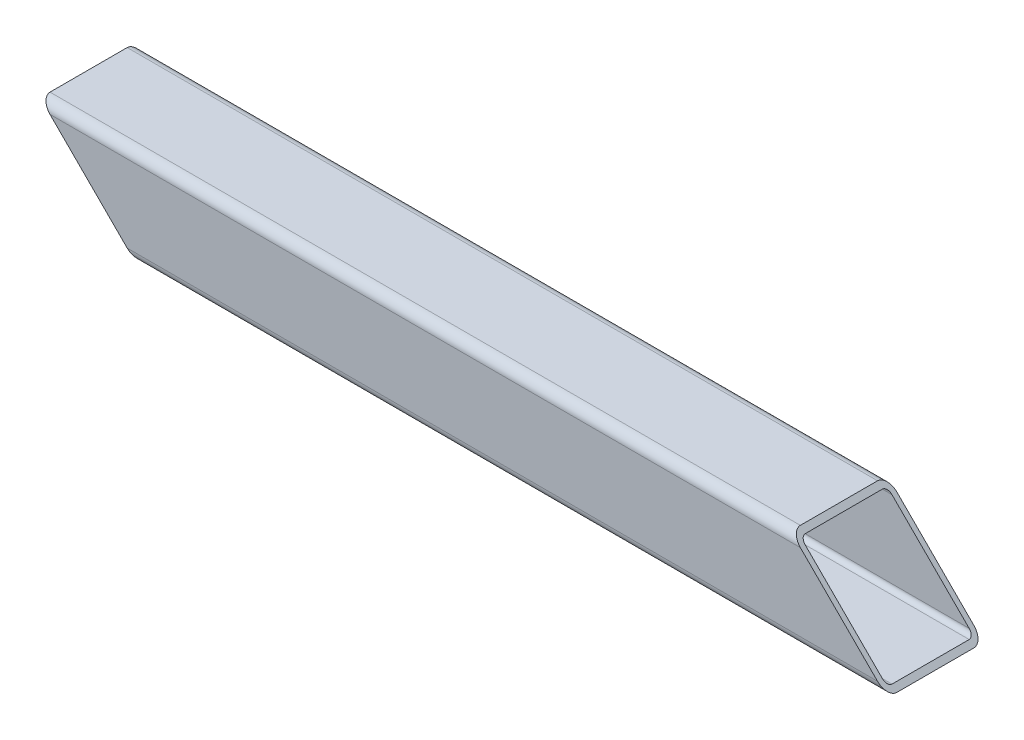
from build123d import *

# Parameters (mm, degrees)
F_100_X_100_X_5_1_DEPTH = 900
CUT_EXTRUDE_1_DEPTH     = 100


with BuildPart() as part:
    # Sketch1 → 方形管 100 X 100 X 5(1) (new body)
    with BuildSketch(Plane(origin=(0, 0, 0), x_dir=(0, 0, -1), z_dir=(1, 0, 0))):
        with BuildLine():
            Line((-40, -50), (40, -50))
            ThreePointArc((40, -50), (47.071067812, -47.071067812), (50, -40))
            Line((50, -40), (50, 40))
            ThreePointArc((50, 40), (47.071067812, 47.071067812), (40, 50))
            Line((40, 50), (-40, 50))
            ThreePointArc((-40, 50), (-47.071067812, 47.071067812), (-50, 40))
            Line((-50, 40), (-50, -40))
            ThreePointArc((-50, -40), (-47.071067812, -47.071067812), (-40, -50))
        make_face()
        with BuildLine():
            Line((-40, -45), (40, -45))
            ThreePointArc((40, -45), (43.535533906, -43.535533906), (45, -40))
            Line((45, -40), (45, 40))
            ThreePointArc((45, 40), (43.535533906, 43.535533906), (40, 45))
            Line((40, 45), (-40, 45))
            ThreePointArc((-40, 45), (-43.535533906, 43.535533906), (-45, 40))
            Line((-45, 40), (-45, -40))
            ThreePointArc((-45, -40), (-43.535533906, -43.535533906), (-40, -45))
        make_face(mode=Mode.SUBTRACT)
    extrude(amount=F_100_X_100_X_5_1_DEPTH)

    # 草图2 → 切除-拉伸1 (cut)
    with BuildSketch(Plane.XY.offset(50)):
        Polygon((0, 50), (100, -50), (0, -50), align=None)
        Polygon((913.789188304, -85.971728999), (913.789188304, 50), (777.817459305, 50), align=None)
    extrude(amount=-CUT_EXTRUDE_1_DEPTH, mode=Mode.SUBTRACT)


solid = part.part
